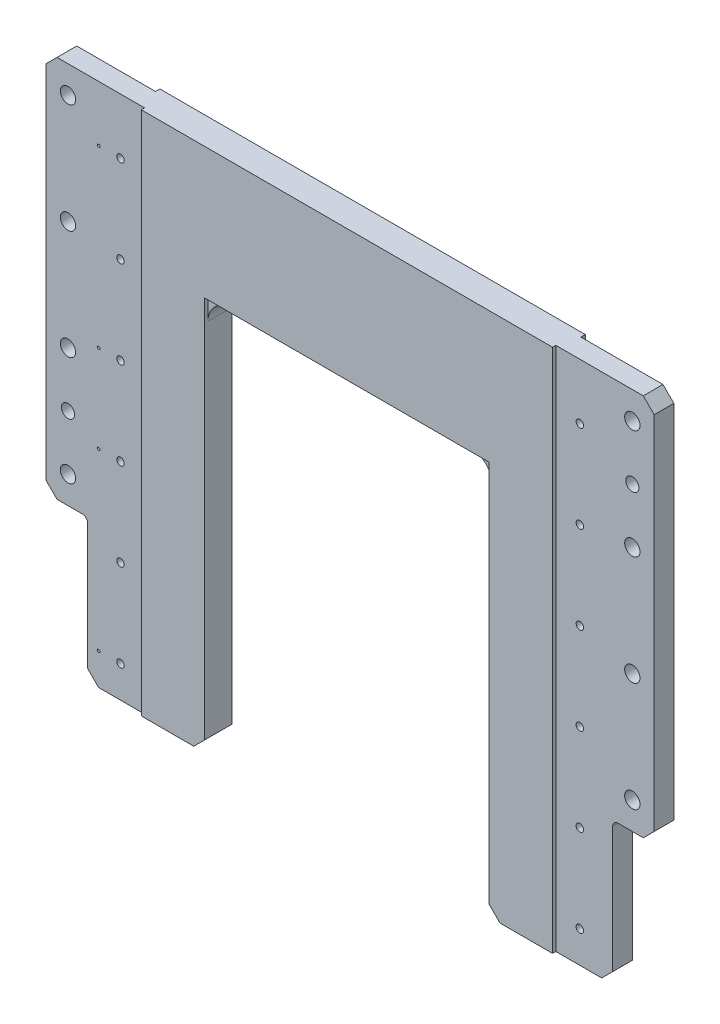
SolidWorks part; units mm, degrees
ref_plane "Front Plane" through (0, 0, 0) normal (0, 0, 1) x (1, 0, 0)
ref_plane "Top Plane" through (0, 0, 0) normal (0, 1, 0) x (1, 0, 0)
ref_plane "Right Plane" through (0, 0, 0) normal (1, 0, 0) x (0, 0, -1)
sketch "Sketch1" plane through (0, 0, 0) normal (0, 0, 1) x (1, 0, 0)
  line L0 (0, 10) -> (0, 470)
  line L1 (10, 480) -> (546, 480)
  line L2 (556, 470) -> (556, 10)
  line L3 (546, 0) -> (418, 0)
  line L4 (148, 10) -> (148, 340)
  line L5 (168, 360) -> (388, 360)
  line L6 (408, 340) -> (408, 10)
  line L7 (138, 0) -> (10, 0)
  line L8 (148, 10) -> (138, 0)
  line L9 (10, 0) -> (0, 10)
  line L10 (418, 0) -> (408, 10)
  line L11 (556, 10) -> (546, 0)
  line L12 (546, 480) -> (556, 470)
  line L13 (0, 470) -> (10, 480)
  arc A0 (408, 340) -> (388, 360) centre (388, 340) ccw
  arc A1 (168, 360) -> (148, 340) centre (168, 340) ccw
  point P0 (0, 0)
  point P1 (0, 480)
  point P4 (556, 480)
  point P5 (556, 0)
  point P6 (148, 0)
  point P9 (408, 0)
  dimension "D6" = 20
  dimension "D1" = 556
  dimension "D2" = 148
  dimension "D3" = 260
  dimension "D4" = 480
  dimension "D5" = 360
extrude "Boss-Extrude1" add sketch "Sketch1" along normal blind 22
sketch "Sketch2" plane through (0, 0, 0) normal (0, 0, -1) x (-1, 0, 0)
  line L0 (-556, 480) -> (-471, 480)
  line L1 (-546, 480) -> (-10, 480) construction
  line L2 (-471, 480) -> (-471, 0)
  line L3 (-418, 0) -> (-546, 0) construction
  line L4 (-471, 0) -> (-556, 0)
  line L5 (-556, 0) -> (-556, 480)
  line L6 (0, 0) -> (-82, 0)
  line L7 (-10, 0) -> (-138, 0) construction
  line L8 (-82, 0) -> (-82, 480)
  line L9 (-82, 480) -> (0, 480)
  line L10 (0, 480) -> (0, 0)
  line L11 (-556, 10) -> (-556, 470) construction
  dimension "D1" = 85
  dimension "D2" = 82
extrude "Cut-Extrude1" cut sketch "Sketch2" against normal blind 4
hole_wizard "M8 Tapped Hole1" positions "3DSketch1" profile "Sketch3" tap size "M8" standard "ISO"
sketch3d "3DSketch1"
  line L0 (546, 0, 4) -> (471, 0, 4) construction
  point P0 (488, 349, 4)
  point P2 (488, 269, 4)
  point P4 (488, 189, 4)
  point P6 (488, 109, 4)
  point P8 (488, 29, 4)
  point P13 (488, 429, 4)
  dimension "D1" = 29
  dimension "D2" = 80
  dimension "D3" = 80
  dimension "D4" = 80
  dimension "D5" = 80
  dimension "D6" = 80
  dimension "D7" = 17
sketch "Sketch3" plane through (488, 349, 4) normal (1, 0, 0) x (0, 1, 0)
  line L0 (0, 0) -> (0, 21.713)
  line L1 (0, 21.713) -> (3.4, 19.75)
  line L2 (3.4, 19.75) -> (3.4, 0)
  line L5 (3.4, 0) -> (0, 0)
  line L10 (0, 21.713) -> (-3.4, 19.75) construction
  line L11 (0, -6.35) -> (0, 107.95) construction
  dimension "Tap Drill Dia." = 6.8
  dimension "Tap Drill Depth" = 19.75
  dimension "Drill Angle" = 120
cosmetic thread "Hole Thread1" parameters "D1"=16, "D2"=8
cosmetic thread "Hole Thread2" parameters "D1"=16, "D2"=8
cosmetic thread "Hole Thread3" parameters "D1"=16, "D2"=8
cosmetic thread "Hole Thread4" parameters "D1"=16, "D2"=8
cosmetic thread "Hole Thread5" parameters "D1"=16, "D2"=8
cosmetic thread "Hole Thread6" parameters "D1"=16, "D2"=8
ref_plane "Plane3" [suppressed] through (278, 0, 0) normal (1, 0, 0) x (0, 0, -1)
ref_plane "Plane4" through (278, 0, 0) normal (-1, 0, 0) x (0, 0, 1)
mirror "Mirror1" about plane through (278, 0, 0) normal (1, 0, 0) of "M8 Tapped Hole1"
hole_wizard "Ø14.0 (14) Diameter Hole1" positions "3DSketch2" profile "Sketch4" hole size "Ø14.0" standard "ISO" end condition up to next
sketch3d "3DSketch2"
  line L0 (556, 470, 4) -> (556, 10, 4) construction
  line L1 (471, 480, 4) -> (546, 480, 4) construction
  point P0 (536, 455, 4)
  point P2 (536, 355, 4)
  point P4 (536, 255, 4)
  point P6 (536, 155, 4)
  dimension "D1" = 20
  dimension "D2" = 25
  dimension "D3" = 100
  dimension "D4" = 100
  dimension "D5" = 100
sketch "Sketch4" plane through (536, 455, 4) normal (1, 0, 0) x (0, 1, 0)
  line L0 (0, 0) -> (0, 18.001)
  line L1 (0, 18.001) -> (7, 18.001)
  line L2 (7, 18.001) -> (7, 0)
  line L5 (7, 0) -> (0, 0)
  line L11 (0, -6.35) -> (0, 107.95) construction
  dimension "Thru Hole Dia." = 14
  dimension "Thru Hole Depth" = 18.001
mirror "Mirror2" about plane through (278, 0, 0) normal (-1, 0, 0) of "Ø14.0 (14) Diameter Hole1"
hole_wizard "Ø7.0 (7) Diameter Hole1" positions "3DSketch3" profile "Sketch5" hole size "Ø7.0" standard "ISO"
sketch3d "3DSketch3"
  line L4 (82, 480, 4) -> (82, 0, 4) construction
  line L5 (82, 0, 4) -> (10, 0, 4) construction
  point P15 (48, 429, 4)
  point P17 (48, 269, 4)
  point P19 (48, 189, 4)
  point P21 (48, 29, 4)
  dimension "D6" = 34
  dimension "D7" = 29
  dimension "D8" = 160
  dimension "D9" = 80
  dimension "D10" = 160
sketch "Sketch5" plane through (48, 429, 4) normal (1, 0, 0) x (0, 1, 0)
  line L0 (0, 0) -> (0, 4)
  line L1 (0, 4) -> (3.5, 4)
  line L2 (3.5, 4) -> (3.5, 0)
  line L5 (3.5, 0) -> (0, 0)
  line L10 (0, 4) -> (-3.5, 4) construction
  line L11 (0, -6.35) -> (0, 107.95) construction
  dimension "Hole Dia." = 7
  dimension "Hole Depth" = 4
  dimension "Drill Angle" = 180
hole_wizard "M3 Tapped Hole1" positions "3DSketch4" profile "Sketch6" tap size "M3" standard "ISO" end condition up to next
sketch3d "3DSketch4"
  line L4 (48, 429, 8) -> (48, 429, 4) construction
  line L5 (48, 269, 8) -> (48, 269, 4) construction
  line L6 (48, 189, 8) -> (48, 189, 4) construction
  line L7 (48, 29, 8) -> (48, 29, 4) construction
  point P16 (48, 429, 4)
  point P20 (48, 269, 8)
  point P24 (48, 189, 4)
  point P28 (48, 29, 8)
sketch "Sketch6" plane through (48, 429, 4) normal (1, 0, 0) x (0, 1, 0)
  line L0 (0, 0) -> (0, 18)
  line L1 (0, 18) -> (1.25, 18)
  line L2 (1.25, 18) -> (1.25, 0)
  line L5 (1.25, 0) -> (0, 0)
  line L11 (0, -6.35) -> (0, 107.95) construction
  dimension "Thru Tap Drill Dia." = 2.5
  dimension "Thru Tap Drill Depth" = 18
cosmetic thread "Hole Thread7" parameters "D2"=3
cosmetic thread "Hole Thread8" parameters "D2"=3
cosmetic thread "Hole Thread9" parameters "D2"=3
cosmetic thread "Hole Thread10" parameters "D2"=3
hole_wizard "Ø12.0 (12) Diameter Hole1" positions "3DSketch5" profile "Sketch8" hole size "Ø12.0" standard "ISO" end condition up to next
sketch3d "3DSketch5"
  line L1 (0, 10, 4) -> (0, 470, 4) construction
  line L3 (471, 480, 4) -> (546, 480, 4) construction
  line L5 (556, 470, 4) -> (556, 10, 4) construction
  circle A0 centre (20, 155, 4) radius 7 construction
  point P3 (20, 205, 4)
  point P12 (20, 155, -3)
  point P28 (536, 405, 4)
  dimension "D1" = 75
  dimension "D2" = 20
  dimension "D3" = 50
  dimension "D4" = 20
sketch "Sketch8" plane through (20, 205, 4) normal (1, 0, 0) x (0, 1, 0)
  line L0 (0, 0) -> (0, 18)
  line L1 (0, 18) -> (6, 18)
  line L2 (6, 18) -> (6, 0)
  line L5 (6, 0) -> (0, 0)
  line L11 (0, -6.35) -> (0, 107.95) construction
  dimension "Thru Hole Dia." = 12
  dimension "Thru Hole Depth" = 18
sketch "Sketch9" plane through (0, 0, 4) normal (0, 0, -1) x (-1, 0, 0)
  line L0 (-556, 0) -> (-518, 0)
  line L1 (-546, 0) -> (-471, 0) construction
  line L2 (-518, 0) -> (-518, 130)
  line L3 (-518, 130) -> (-556, 130)
  line L4 (-556, 470) -> (-556, 10) construction
  line L5 (-556, 130) -> (-556, 0)
  line L6 (-278, 559.5128) -> (-278, 78.7074) construction
  line L8 (-278, -9.9) -> (-278, 9.9) construction
  line L9 (0, 130) -> (0, 0)
  line L10 (-38, 130) -> (0, 130)
  line L11 (-38, 0) -> (-38, 130)
  line L12 (0, 0) -> (-38, 0)
  dimension "D1" = 38
  dimension "D2" = 130
extrude "Cut-Extrude2" cut sketch "Sketch9" against normal up to next and the other way blind 5
fillet "Fillet1" radius 5 2 edges at (38, 130, 13) (518, 130, 13)
chamfer "Chamfer1" distance 10 angle 45 4 edges at (0, 130, 13) (38, 0, 13) (518, 0, 13) (556, 130, 13)
sketch "Sketch10" plane through (0, 0, 22) normal (0, 0, 1) x (1, 0, 0)
  line L0 (90, 480) -> (90, 0)
  line L1 (546, 480) -> (10, 480) construction
  line L2 (48, 0) -> (138, 0) construction
  line L3 (90, 0) -> (138, 0)
  line L4 (138, 0) -> (148, 10)
  line L5 (148, 10) -> (148, 360)
  line L6 (148, 360) -> (408, 360)
  line L7 (408, 360) -> (408, 10)
  line L8 (408, 340) -> (408, 10) construction
  line L9 (408, 10) -> (418, 0)
  line L10 (418, 0) -> (466, 0)
  line L12 (418, 0) -> (508, 0) construction
  line L13 (466, 0) -> (466, 480)
  line L14 (466, 480) -> (90, 480)
  line L15 (0, 470) -> (0, 140) construction
  line L16 (556, 140) -> (556, 470) construction
  dimension "D1" = 90
  dimension "D2" = 90
extrude "Boss-Extrude2" add sketch "Sketch10" along normal blind 3
